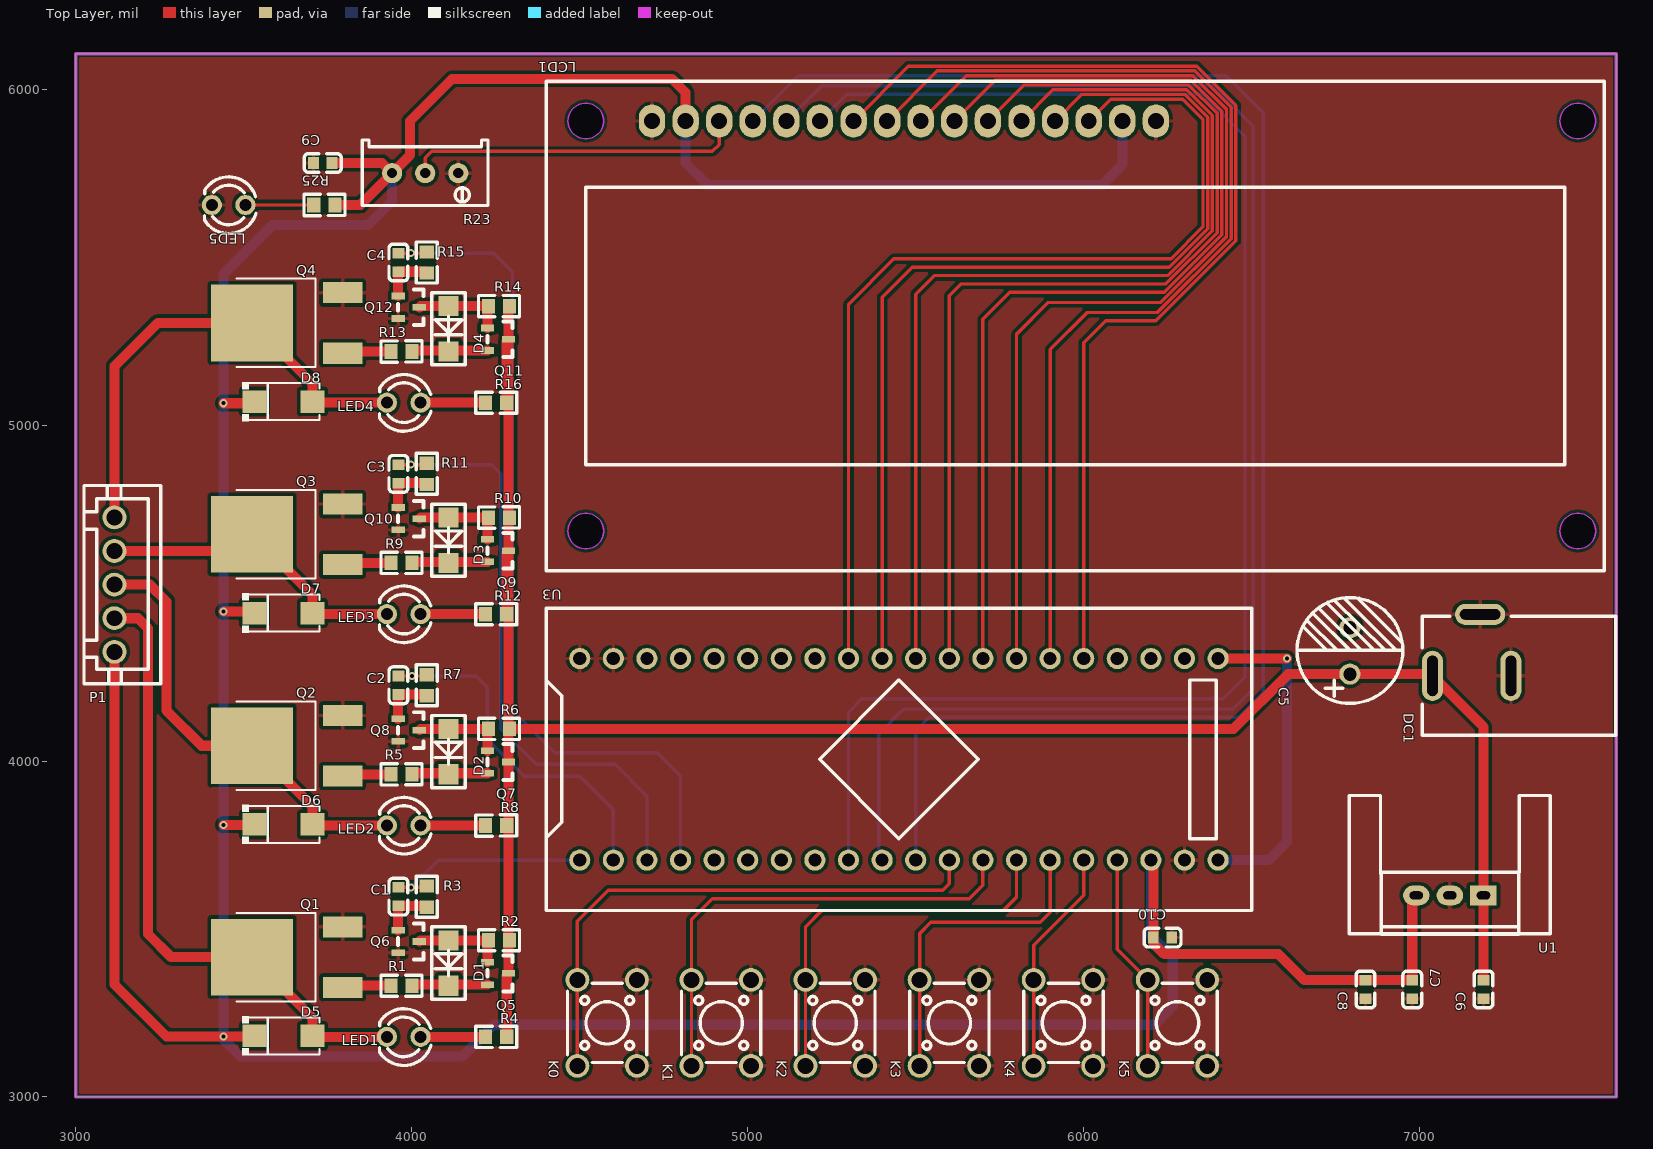
[diagram p0: Top Layer view]
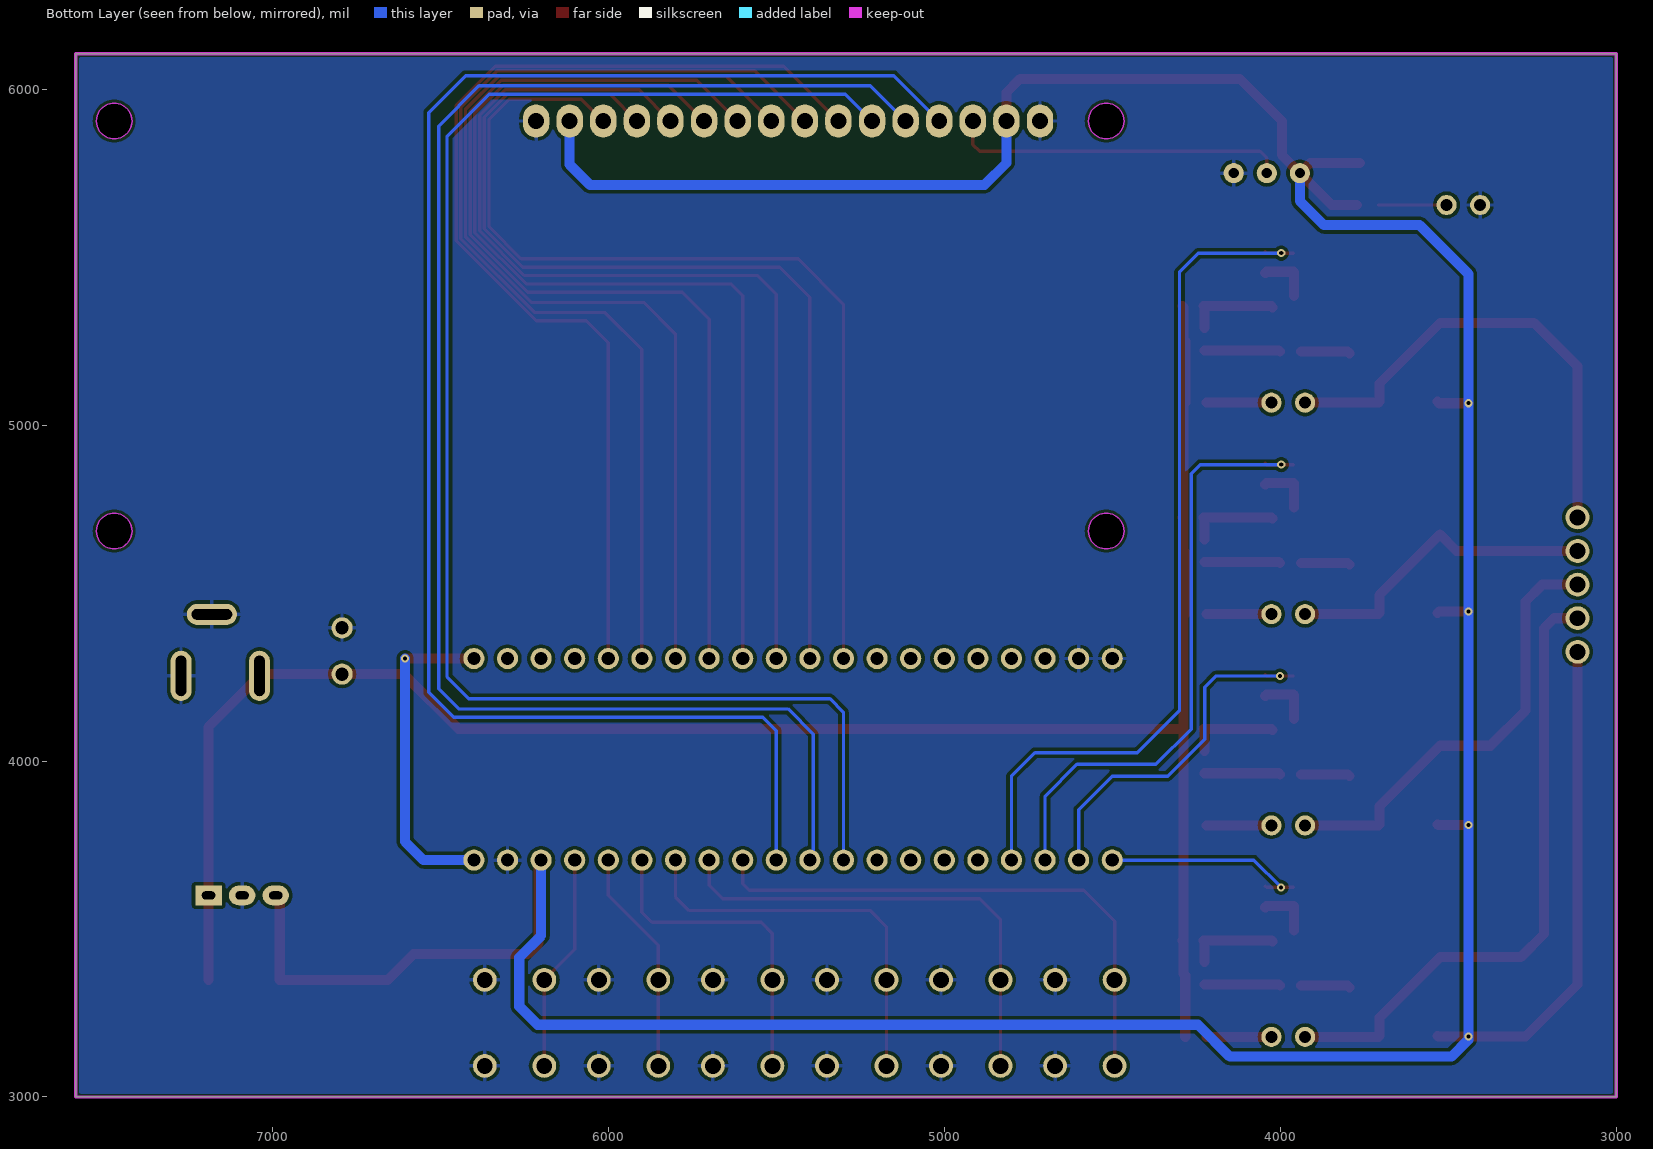
[diagram p1: Bottom Layer view, seen from below]
# Altium PCB MISC49935.pcbdoc
Units mil, origin at the board's own origin, x right, y up, seen from the top; angles counter-clockwise.
Board outline 4585 x 3105 mil, 2 copper layers (Top Layer, Bottom Layer), stack 62.206 mil thick; 64 components, 64 nets, 210 pads, 9 vias.

## Layer stack, top to bottom
Top Solder Mask Layer: solder mask 0.394, Dk 3.3
Top Layer: signal copper 1.379
Dielectric1: surface 59.449, FR4, Dk 4.5
Bottom Layer: signal copper 1.378
Bottom Solder Mask Layer: solder mask 0.394, Dk 3.3

## Board outline
3000,6105 3000,3000 7585,3000 7585,6105

## Design rules (kind name [scope] priority, off if disabled: settings)
BoardOutlineClearance copperThickness2oz_1 [All] p2 off: genericclearance=7.99 ignorepadtopadclearanceinfootprint=FALSE except(0: Arc-SplitContinuation Track-SplitContinuation SMDPad-SplitContinuation THPad-SplitContinuation Via-SplitContinuation Fill-SplitContinuation Region-SplitContinuation Poly-SplitContinuation Text-SplitContinuation Hole-SplitContinuation; 5.98: Arc-CutoutEdge SMDPad-CutoutEdge THPad-CutoutEdge Via-CutoutEdge Fill-CutoutEdge Region-CutoutEdge Text-CutoutEdge; 6.93: Hole-OutlineEdge Hole-CutoutEdge; 10: Poly-OutlineEdge Poly-CutoutEdge; 11.81: Arc-OutlineEdge Track-OutlineEdge SMDPad-OutlineEdge THPad-OutlineEdge Via-OutlineEdge Fill-OutlineEdge Region-OutlineEdge Text-OutlineEdge Track-CutoutEdge)
BoardOutlineClearance copperThickness1oz_1 [All] p4: genericclearance=4.02 ignorepadtopadclearanceinfootprint=FALSE except(0: Arc-SplitContinuation Track-SplitContinuation SMDPad-SplitContinuation THPad-SplitContinuation Via-SplitContinuation Fill-SplitContinuation Region-SplitContinuation Poly-SplitContinuation Text-SplitContinuation Hole-SplitContinuation; 6: SMDPad-CutoutEdge THPad-CutoutEdge Via-CutoutEdge Fill-CutoutEdge Region-CutoutEdge Text-CutoutEdge; 6.93: Hole-OutlineEdge Hole-CutoutEdge; 10: Poly-OutlineEdge Poly-CutoutEdge; 11.8: Arc-OutlineEdge Track-OutlineEdge SMDPad-OutlineEdge THPad-OutlineEdge Via-OutlineEdge Fill-OutlineEdge Region-OutlineEdge Text-OutlineEdge; 11.81: Arc-CutoutEdge Track-CutoutEdge)
Clearance copperThickness2oz [All] p1 off: gap=7.99 ignorepadtopadclearanceinfootprint=FALSE except(5.98: SMDPad-Track SMDPad-SMDPad THPad-Track SMDPad-THPad THPad-THPad Track-Via SMDPad-Via THPad-Via Via-Via Fill-Track Region-Track Fill-SMDPad Region-SMDPad Fill-THPad Region-THPad Fill-Via Region-Via Fill-Fill Fill-Region Region-Region Arc-Track Arc-SMDPad Arc-THPad Arc-Via Fill-Arc Region-Arc Arc-Arc Text-Track SMDPad-Text Text-THPad Text-Via Fill-Text Region-Text Arc-Text Text-Text; 6.93: Hole-Track Hole-SMDPad Hole-THPad Hole-Via Fill-Hole Region-Hole Hole-Arc Hole-Text; 10: Poly-Track Poly-SMDPad Poly-THPad Poly-Via Poly-Fill Poly-Region Poly-Poly Poly-Arc Poly-Text Poly-Hole)
Clearance copperThickness1oz [All] p3: gap=4.02 ignorepadtopadclearanceinfootprint=FALSE except(5.98: SMDPad-Track SMDPad-SMDPad THPad-Track SMDPad-THPad THPad-THPad Track-Via SMDPad-Via THPad-Via Via-Via Fill-Track Region-Track Fill-SMDPad Region-SMDPad Fill-THPad Region-THPad Fill-Via Region-Via Fill-Fill Fill-Region Region-Region; 6: Arc-Track Arc-SMDPad Arc-THPad Arc-Via Fill-Arc Region-Arc Arc-Arc Text-Track SMDPad-Text Text-THPad Text-Via Fill-Text Region-Text Arc-Text Text-Text; 6.93: Hole-Track Hole-SMDPad Hole-THPad Hole-Via Fill-Hole Region-Hole Hole-Arc Hole-Text; 10: Poly-Track Poly-SMDPad Poly-THPad Poly-Via Poly-Fill Poly-Region Poly-Poly Poly-Arc Poly-Text Poly-Hole)
Creepage creepage [All] p1: checkdistance=0 ignoreinternallayers=TRUE applytopolygonpour=TRUE
DiffPairsRouting differentialPair [All] p1: maxlimit=6 minlimit=6 mostfreqgap=6 toplayer_minwidth=5 toplayer_prefwidth=10 toplayer_maxwidth=100 toplayer_mingap=6 toplayer_prefgap=6 toplayer_maxgap=6 bottomlayer_minwidth=5 bottomlayer_prefwidth=10 bottomlayer_maxwidth=100 bottomlayer_mingap=6 bottomlayer_prefgap=6 bottomlayer_maxgap=6 maxuncoupledlength=10
HoleToHoleClearance otherClearance [All] p1: gap=11.81 allowstackedmicrovias=TRUE
Length netLength [All] p1: minlimit=0 maxlimit=0
MatchedLengths netLengthTolerance [All] p1: tolerance=1000
PasteMaskExpansion pasteMaskExpansion [All] p1: expansion=0
PlaneConnect innerPlane [All] p1: planeconnectstyle=Relief reliefexpansion=20 reliefentries=4 reliefconductorwidth=10 reliefairgap=10
PolygonConnect copperRegion [(InNet('GND'))] p1: connectstyle=Relief reliefconductorwidth=10 reliefentries=4 polygonreliefangle="90 Angle" airgapwidth=10 via.connectstyle=Relief via.reliefconductorwidth=10 via.reliefentries=4 via.polygonreliefangle="90 Angle" via.airgapwidth=10
RoutingVias viaSize [All] p1: holewidth=12.01 width=24.02 viastyle="Through Hole" minholewidth=11.81 minwidth=19.68 maxholewidth=248.03 maxwidth=393.7
SolderMaskExpansion solderMaskExpansion [IsVia] p1: expansion=-1000 istentingtop=TRUE
SolderMaskExpansion solderMaskExpansion [All] p2: expansion=2 istentingtop=FALSE
Width copperThickness2oz_2 [All] p1 off: maxlimit=100 minlimit=8 preferedwidth=10
Width copperThickness1oz_2 [All] p2: maxlimit=100 minlimit=5 preferedwidth=10

## Components (designator, comment, footprint, x,y, rotation, side; value= is the part's Value field where it differs from the comment)
C1 "1nF" C0603 3960.27,3596.17 r270 top
C2 "1nF" C0603 3960.27,4225.43 r270 top
C3 "1nF" C0603 3960.27,4854.68 r270 top
C4 "1nF" C0603 3960.27,5483.94 r270 top
C5 "470uF" 470uf 6795,4330 r90 top
C6 "100nF" C0603 7190,3320 r90 top
C7 "100uF" C0603 6978.03,3320 r270 top
C8 "100nF" C0603 6838.9,3320 r90 top
C9 "100nF" C0603 3735,5780 r0 top
C10 "100nF" C0603 6234.77,3474.49 r0 top
D1 "1N4148" 1N4148 4109.51,3401.21 r270 top
D2 "1N4148" 1N4148 4109.51,4030.47 r270 top
D3 "1N4148" 1N4148 4109.51,4659.72 r270 top
D4 "1N4148" 1N4148 4109.51,5288.98 r270 top
D5 "1N4007G" 1N4007G/M7 3616.09,3178.82 r0 top
D6 "1N4007G" 1N4007G/M7 3616.09,3808.08 r0 top
D7 "1N4007G" 1N4007G/M7 3616.09,4437.33 r0 top
D8 "1N4007G" 1N4007G/M7 3616.09,5066.59 r0 top
DC1 "EJ503A" DC-IN-TH_EJ503A 7155,4345 r90 top
K0 "Start/Stop" SW-TH_4P-L6.0-W6.0-P4.50-LS6.5 4581.56,3220.54 r90 top
K1 "Forward/Reverse" SW-TH_4P-L6.0-W6.0-P4.50-LS6.5 4921.09,3220.54 r90 top
K2 "Speed+10" SW-TH_4P-L6.0-W6.0-P4.50-LS6.5 5260.61,3220.54 r90 top
K3 "Speed+1" SW-TH_4P-L6.0-W6.0-P4.50-LS6.5 5600.14,3220.54 r90 top
K4 "Speed-10" SW-TH_4P-L6.0-W6.0-P4.50-LS6.5 5939.66,3220.54 r90 top
K5 "Speed-1" SW-TH_4P-L6.0-W6.0-P4.50-LS6.5 6279.19,3220.54 r90 top
LCD1 "LCM1602K-FSW-FBW-33V33" MODULE-TH_LCM1602K 5465,5905 r0 top
LED1 "3mmFIR" LED_TH-3mm 3976.09,3178.82 r180 top
LED2 "3mmFIR" LED_TH-3mm 3976.09,3808.08 r180 top
LED3 "3mmFIR" LED_TH-3mm 3976.09,4437.33 r180 top
LED4 "3mmFIR" LED_TH-3mm 3976.09,5066.59 r180 top
LED5 "3mmFIR" LED_TH-3mm 3455,5655 r180 top
P1 "Motor interface" CONN-TH_5P-P2.54_C9900008095 3115,4525 r90 top
Q1 "JSM80N03D" TO-252-2_L6.6-W6.1-P4.57-LS9.9-BR-CW 3659.51,3416.21 r0 top
Q2 "JSM80N03D" TO-252-2_L6.6-W6.1-P4.57-LS9.9-BR-CW 3659.51,4045.47 r0 top
Q3 "JSM80N03D" TO-252-2_L6.6-W6.1-P4.57-LS9.9-BR-CW 3659.51,4674.72 r0 top
Q4 "JSM80N03D" TO-252-2_L6.6-W6.1-P4.57-LS9.9-BR-CW 3659.51,5303.98 r0 top
Q5 "MMS9013-H-TP" MMS8050-H-TP 4225.27,3401.17 r270 top
Q6 "MMS9013-H-TP" MMS8050-H-TP 3959.51,3496.21 r270 top
Q7 "MMS9013-H-TP" MMS8050-H-TP 4225.27,4030.43 r270 top
Q8 "MMS9013-H-TP" MMS8050-H-TP 3959.51,4125.47 r270 top
Q9 "MMS9013-H-TP" MMS8050-H-TP 4225.27,4659.68 r270 top
Q10 "MMS9013-H-TP" MMS8050-H-TP 3959.51,4754.72 r270 top
Q11 "MMS9013-H-TP" MMS8050-H-TP 4225.27,5288.94 r270 top
Q12 "MMS9013-H-TP" MMS8050-H-TP 3959.51,5383.98 r270 top
R1 "5.1Ω" R0603 3969.51,3331.21 r180 top
R2 "10kΩ" R0603 4259.51,3466.21 r0 top
R3 "1kΩ" R0603 4044.51,3596.21 r270 top
R4 "10kΩ" R0603 4251.09,3178.82 r180 top
R5 "5.1Ω" R0603 3969.51,3960.47 r180 top
R6 "10kΩ" R0603 4259.51,4095.47 r0 top
R7 "1kΩ" R0603 4044.51,4225.47 r270 top
R8 "10kΩ" R0603 4251.09,3808.08 r180 top
R9 "5.1Ω" R0603 3969.51,4589.72 r180 top
R10 "10kΩ" R0603 4259.51,4724.72 r0 top
R11 "1kΩ" R0603 4044.51,4854.72 r270 top
R12 "10kΩ" R0603 4251.09,4437.33 r180 top
R13 "5.1Ω" R0603 3969.51,5218.98 r180 top
R14 "10kΩ" R0603 4259.51,5353.98 r0 top
R15 "1kΩ" R0603 4044.51,5483.98 r270 top
R16 "10kΩ" R0603 4251.09,5066.59 r180 top
R23 "10kΩ" R_3296 4040,5745 r180 top
R25 "3kΩ" R0603 3740,5655 r0 top
U1 "LM7805" LM7805 7090,3600 r180 top
U3 "LCKFB-DKX-STM32F103C8T6" CONN-TH_L53.3-W22.9_STM32F103C8T6-CARD 5450,4005 r0 top

## Footprints (in the part's own frame and the unit in brackets; to place one, negate y for a bottom-side part, rotate by r counter-clockwise, add the part's x,y. Pads: shape width x height; smd on the part's side, far side on the other; paste and mask are expansions set on the pad)
1N4007G/M7 [mm]
  rect 1.8x1.7 smd paste+0 mask+0.102: 1(-2.133,0.081) 2(2.252,0.081)
  silkscreen extent -3.05,-1.4 2.79,1.56
1N4148 [mil]
  rect 60x60 smd paste+0 mask+4: 1(70,0) 2(-65,0)
  silkscreen extent -105,-50 110,50
470uf [mm]
  round 1.6 hole 1 paste+0 mask+0.051: 1(-1.814,0.062) 2(1.686,0.062)
  silkscreen extent -4.03,-3.94 3.97,4.06
C0603 [mm]
  rect 0.8x0.9 smd: 1(-0.7,0) 2(0.7,0)
  silkscreen extent -1.39,-0.71 1.39,0.71
CONN-TH_5P-P2.54_C9900008095 [mm]
  round 1.8 hole 1.2 paste+0 mask+0.05: 1(-5.08,0) 2(-2.54,0) 3(0,0) 5(5.08,0)
  round 1.8 hole 1.2 copper offset 0,0 paste+0 mask+0.05: 4(2.54,0)
  silkscreen extent -7.5,-3.5 7.5,2.3
CONN-TH_L53.3-W22.9_STM32F103C8T6-CARD [mm]
  round 1.6 hole 1: 1(-24.13,-7.62) 2(-21.59,-7.62) 3(-19.05,-7.62) 4(-16.51,-7.62) 5(-13.97,-7.62) 6(-11.43,-7.62) 7(-8.89,-7.62) 8(-6.35,-7.62) 9(-3.81,-7.62) 10(-1.27,-7.62) 11(1.27,-7.62) 12(3.81,-7.62) 13(6.35,-7.62) 14(8.89,-7.62) 15(11.43,-7.62) 16(13.97,-7.62) 17(16.51,-7.62) 18(19.05,-7.62) 19(21.59,-7.62) 20(24.13,-7.62) 21(24.13,7.62) 22(21.59,7.62) 23(19.05,7.62) 24(16.51,7.62) 25(13.97,7.62) 26(11.43,7.62) 27(8.89,7.62) 28(6.35,7.62) 29(3.81,7.62) 30(1.27,7.62) 31(-1.27,7.62) 32(-3.81,7.62) 33(-6.35,7.62) 34(-8.89,7.62) 35(-11.43,7.62) 36(-13.97,7.62) 37(-16.51,7.62) 38(-19.05,7.62) 39(-21.59,7.62) 40(-24.13,7.62)
  silkscreen extent -26.67,-11.43 26.67,11.43
DC-IN-TH_EJ503A [mm]
  oval 3.8x1.6 hole 0.8 slot 3.05 at 0 deg paste+0 mask+0.05: 1(-2.325,2.965) 2(-2.325,-2.965)
  oval 1.6x3.8 hole 0.8 slot 3.05 at 90 deg copper offset 0,0 paste+0 mask+0.05: 3(2.325,-0.635)
  silkscreen extent -6.82,-10.89 2.18,3.73
LED_TH-3mm [mil]
  round 60 hole 36 paste+0 mask+2: 1(-50,0) 2(50,0)
  silkscreen extent -81,-84 72,85
LM7805 [mm]
  rect 2x1.5 hole 0.6 slot 1 at 0 deg: 1(-2.54,0)
  oval 2x1.5 hole 0.6 slot 1 at 0 deg: 2(0,0) 3(2.54,0)
  silkscreen extent -7.6,-7.55 7.6,2.95
MMS8050-H-TP [mm]
  rect 0.5x1 smd paste+0 mask+0.102: 1(0,0) 2(1.7,0) 3(0.85,1.6)
  silkscreen extent -0.5,0 2.2,1.9
MODULE-TH_LCM1602K [mm]
  oval 2x2.5 hole 1.2: 1(-19.05,0) 2(-16.51,0) 3(-13.97,0) 4(-11.43,0) 5(-8.89,0) 6(-6.35,0) 7(-3.81,0) 8(-1.27,0) 9(1.27,0) 10(3.81,0) 11(6.35,0) 12(8.89,0) 13(11.43,0) 14(13.97,0) 15(16.51,0) 16(19.05,0)
  Board Outline Layer circle w0.003: c-24.051,0 r1.35
  Board Outline Layer circle w0.003: c50.95,0 r1.35
  Board Outline Layer circle w0.003: c50.95,-31.001 r1.35
  Board Outline Layer circle w0.003: c-24.051,-31.001 r1.35
  Board Outline Layer region: -22.701,0 -22.835,-0.586 -23.21,-1.055 -23.751,-1.316 -24.352,-1.316 -24.893,-1.055 -25.268,-0.586 -25.401,0 -25.401,0 -25.268,0.586 -24.893,1.055 -24.352,1.316 -23.751,1.316 -23.21,1.055 -22.835,0.586 -22.701,0
  Board Outline Layer region: -22.701,0 -22.711,-0.163 -22.74,-0.323 -22.789,-0.479 -22.856,-0.627 -22.94,-0.767 -23.041,-0.895 -23.156,-1.01 -23.284,-1.111 -23.424,-1.195 -23.573,-1.262 -23.728,-1.311 -23.889,-1.34 -24.051,-1.35 -24.214,-1.34 -24.374,-1.311 -24.53,-1.262 -24.679,-1.195 -24.818,-1.111 -24.946,-1.01 -25.062,-0.895 -25.162,-0.767 -25.247,-0.627 -25.314,-0.479 -25.362,-0.323 -25.391,-0.163 -25.401,0 -25.391,0.163 -25.362,0.323 -25.314,0.479 -25.247,0.627 -25.162,0.767 -25.062,0.895 -24.946,1.01 -24.818,1.111 -24.679,1.195 -24.53,1.262 -24.374,1.311 -24.214,1.34 -24.051,1.35 -23.889,1.34 -23.728,1.311 -23.573,1.262 -23.424,1.195 -23.284,1.111 -23.156,1.01 -23.041,0.895 -22.94,0.767 -22.856,0.627 -22.789,0.479 -22.74,0.323 -22.711,0.163
  Board Outline Layer region: 52.3,0 52.166,-0.586 51.792,-1.055 51.25,-1.316 50.649,-1.316 50.108,-1.055 49.734,-0.586 49.6,0 49.6,0 49.734,0.586 50.108,1.055 50.649,1.316 51.25,1.316 51.792,1.055 52.166,0.586 52.3,0
  Board Outline Layer region: 52.3,0 52.29,-0.163 52.261,-0.323 52.212,-0.479 52.145,-0.627 52.061,-0.767 51.96,-0.895 51.845,-1.01 51.717,-1.111 51.577,-1.195 51.429,-1.262 51.273,-1.311 51.113,-1.34 50.95,-1.35 50.787,-1.34 50.627,-1.311 50.471,-1.262 50.322,-1.195 50.183,-1.111 50.055,-1.01 49.939,-0.895 49.839,-0.767 49.754,-0.627 49.688,-0.479 49.639,-0.323 49.61,-0.163 49.6,0 49.61,0.163 49.639,0.323 49.688,0.479 49.754,0.627 49.839,0.767 49.939,0.895 50.055,1.01 50.183,1.111 50.322,1.195 50.471,1.262 50.627,1.311 50.787,1.34 50.95,1.35 51.113,1.34 51.273,1.311 51.429,1.262 51.577,1.195 51.717,1.111 51.845,1.01 51.96,0.895 52.061,0.767 52.145,0.627 52.212,0.479 52.261,0.323 52.29,0.163
  Board Outline Layer region: 52.3,-31.001 52.166,-31.586 51.792,-32.056 51.25,-32.317 50.649,-32.317 50.108,-32.056 49.734,-31.586 49.6,-31.001 49.6,-31.001 49.734,-30.415 50.108,-29.945 50.649,-29.685 51.25,-29.685 51.792,-29.945 52.166,-30.415 52.3,-31.001
  Board Outline Layer region: 52.3,-31.001 52.29,-31.163 52.261,-31.324 52.212,-31.479 52.145,-31.628 52.061,-31.768 51.96,-31.896 51.845,-32.011 51.717,-32.112 51.577,-32.196 51.429,-32.263 51.273,-32.311 51.113,-32.341 50.95,-32.351 50.787,-32.341 50.627,-32.311 50.471,-32.263 50.322,-32.196 50.183,-32.112 50.055,-32.011 49.939,-31.896 49.839,-31.768 49.754,-31.628 49.688,-31.479 49.639,-31.324 49.61,-31.163 49.6,-31.001 49.61,-30.838 49.639,-30.678 49.688,-30.522 49.754,-30.373 49.839,-30.234 49.939,-30.105 50.055,-29.99 50.183,-29.89 50.322,-29.805 50.471,-29.738 50.627,-29.69 50.787,-29.661 50.95,-29.651 51.113,-29.661 51.273,-29.69 51.429,-29.738 51.577,-29.805 51.717,-29.89 51.845,-29.99 51.96,-30.105 52.061,-30.234 52.145,-30.373 52.212,-30.522 52.261,-30.678 52.29,-30.838
  Board Outline Layer region: -22.701,-31.001 -22.835,-31.586 -23.21,-32.056 -23.751,-32.317 -24.352,-32.317 -24.893,-32.056 -25.268,-31.586 -25.401,-31.001 -25.401,-31.001 -25.268,-30.415 -24.893,-29.945 -24.352,-29.685 -23.751,-29.685 -23.21,-29.945 -22.835,-30.415 -22.701,-31.001
  Board Outline Layer region: -22.701,-31.001 -22.711,-31.163 -22.74,-31.324 -22.789,-31.479 -22.856,-31.628 -22.94,-31.768 -23.041,-31.896 -23.156,-32.011 -23.284,-32.112 -23.424,-32.196 -23.573,-32.263 -23.728,-32.311 -23.889,-32.341 -24.051,-32.351 -24.214,-32.341 -24.374,-32.311 -24.53,-32.263 -24.679,-32.196 -24.818,-32.112 -24.946,-32.011 -25.062,-31.896 -25.162,-31.768 -25.247,-31.628 -25.314,-31.479 -25.362,-31.324 -25.391,-31.163 -25.401,-31.001 -25.391,-30.838 -25.362,-30.678 -25.314,-30.522 -25.247,-30.373 -25.162,-30.234 -25.062,-30.105 -24.946,-29.99 -24.818,-29.89 -24.679,-29.805 -24.53,-29.738 -24.374,-29.69 -24.214,-29.661 -24.051,-29.651 -23.889,-29.661 -23.728,-29.69 -23.573,-29.738 -23.424,-29.805 -23.284,-29.89 -23.156,-29.99 -23.041,-30.105 -22.94,-30.234 -22.856,-30.373 -22.789,-30.522 -22.74,-30.678 -22.711,-30.838
  Multi-Layer board cut-out: -22.701,0 -22.835,-0.586 -23.21,-1.055 -23.751,-1.316 -24.352,-1.316 -24.893,-1.055 -25.268,-0.586 -25.401,0 -25.401,0 -25.268,0.586 -24.893,1.055 -24.352,1.316 -23.751,1.316 -23.21,1.055 -22.835,0.586 -22.701,0
  Multi-Layer board cut-out: 52.3,0 52.166,-0.586 51.792,-1.055 51.25,-1.316 50.649,-1.316 50.108,-1.055 49.734,-0.586 49.6,0 49.6,0 49.734,0.586 50.108,1.055 50.649,1.316 51.25,1.316 51.792,1.055 52.166,0.586 52.3,0
  Multi-Layer board cut-out: 52.3,-31.001 52.166,-31.586 51.792,-32.056 51.25,-32.317 50.649,-32.317 50.108,-32.056 49.734,-31.586 49.6,-31.001 49.6,-31.001 49.734,-30.415 50.108,-29.945 50.649,-29.685 51.25,-29.685 51.792,-29.945 52.166,-30.415 52.3,-31.001
  Multi-Layer board cut-out: -22.701,-31.001 -22.835,-31.586 -23.21,-32.056 -23.751,-32.317 -24.352,-32.317 -24.893,-32.056 -25.268,-31.586 -25.401,-31.001 -25.401,-31.001 -25.268,-30.415 -24.893,-29.945 -24.352,-29.685 -23.751,-29.685 -23.21,-29.945 -22.835,-30.415 -22.701,-31.001
  silkscreen extent -27.05,-34 52.95,3
R0603 [mm]
  rect 1x1.1 smd paste+0 mask+0.102: 1(-0.8,0) 2(0.8,0)
  silkscreen extent -1.55,-0.8 1.55,0.81
R_3296 [mil]
  round 60 hole 30 paste+0 mask+2: 1(-98.4,-5) 2(0,-5) 3(98.4,-5)
  silkscreen extent -187,-103 187,92
SW-TH_4P-L6.0-W6.0-P4.50-LS6.5 [mm]
  round 1.8 hole 1.2: 1(-3.25,2.25) 2(3.25,2.25) 3(-3.25,-2.25) 4(3.25,-2.25)
  silkscreen extent -3,-3 3,3
TO-252-2_L6.6-W6.1-P4.57-LS9.9-BR-CW [mm]
  rect 3x1.6 smd: 1(3.424,-2.29) 3(3.424,2.29)
  rect 6.2x5.8 smd: 2(-3.424,0)
  silkscreen extent -4.58,-3.35 1.38,3.35

## Via types
v1: diameter 24.02, hole 12, Top Layer to Bottom Layer, 9 vias

## Nets (pads, with @x,y where several pads share a name; then routed paths per layer and width w, separated by ;. In a path a pad name is that pad's centre, name@x,y a point inside that pad or via, vN(x,y) a via of type N, cw(c..) or ccw(c..) an arc to the next point about the centre after c; other vN are vias at no path point)
$1N1: D6.2 LED2.2 P1.3 Q2.2 | length 1330.2
  Top Layer w30: P1.3 3220,4525 3270,4475 3270,4150 3374.53,4045.47 Q2.2 3704.74,3865.43 D6.2 3707.91,3808.08 LED2.2
$1N3: D5.2 LED1.2 P1.2 Q1.2 | length 1892.1
  Top Layer w30: P1.2 3185,4425 3215,4395 3215,3485 3283.79,3416.21 Q1.2 3704.74,3236.17 D5.2 3707.91,3178.82 LED1.2
$1N6: D7.2 LED3.2 P1.4 Q3.2 | length 961.8
  Top Layer w30: P1.4 3474.99,4625.01 Q3.2 3704.74,4494.68 D7.2 3707.91,4437.33 LED3.2
$1N8: D8.2 LED4.2 P1.5 Q4.2 | length 1444.6
  Top Layer w30: P1.5 3115,5175 3243.98,5303.98 Q4.2 3704.74,5123.94 D8.2 3707.91,5066.59 LED4.2
$1N9: Q1.1 R1.2 | length 145.8
  Top Layer w30: Q1.1 3799.47,3331.21 R1.2
$1N10: LED1.1 R4.2 | length 193.5
  Top Layer w30: LED1.1 R4.2
$1N12: D1.1 Q5.2 R1.1 | length 225.5
  Top Layer w30: R1.1 4004.03,3334.24 Q5.2
$1N13: D1.2 Q5.1 Q6.3 R2.1 | length 273.1
  Top Layer w30: Q6.3 4025.96,3466.21 D1.2 R2.1 4225.27,3463.46 Q5.1
$1N15: C1.2 Q6.1 R3.2 | length 158.6
  Top Layer w30: Q6.1 3959.51,3567.85 C1.2 4040.6,3568.61 R3.2
$1N18: C2.2 Q8.1 R7.2 | length 158.6
  Top Layer w30: Q8.1 3959.51,4197.11 C2.2 4040.6,4197.87 R7.2
$1N20: D2.2 Q7.1 Q8.3 R6.1 | length 273.1
  Top Layer w30: Q8.3 4025.96,4095.47 D2.2 R6.1 4225.27,4092.72 Q7.1
$1N21: D2.1 Q7.2 R5.1 | length 225.5
  Top Layer w30: R5.1 4004.03,3963.5 Q7.2
$1N23: LED2.1 R8.2 | length 193.5
  Top Layer w30: LED2.1 R8.2
$1N24: Q2.1 R5.2 | length 145.8
  Top Layer w30: Q2.1 3799.47,3960.47 R5.2
$1N26: C3.2 Q10.1 R11.2 | length 158.6
  Top Layer w30: Q10.1 3959.51,4826.36 C3.2 4040.6,4827.12 R11.2
$1N28: D3.2 Q9.1 Q10.3 R10.1 | length 273.1
  Top Layer w30: Q10.3 4025.96,4724.72 D3.2 R10.1 4225.27,4721.97 Q9.1
$1N29: D3.1 Q9.2 R9.1 | length 225.5
  Top Layer w30: R9.1 4004.03,4592.75 Q9.2
$1N31: LED3.1 R12.2 | length 193.5
  Top Layer w30: LED3.1 R12.2
$1N32: Q3.1 R9.2 | length 145.8
  Top Layer w30: Q3.1 3799.47,4589.72 R9.2
$1N34: C4.2 Q12.1 R15.2 | length 158.6
  Top Layer w30: Q12.1 3959.51,5455.62 C4.2 4040.6,5456.38 R15.2
$1N36: D4.2 Q11.1 Q12.3 R14.1 | length 273.1
  Top Layer w30: Q12.3 4025.96,5353.98 D4.2 R14.1 4225.27,5351.23 Q11.1
$1N37: D4.1 Q11.2 R13.1 | length 225.5
  Top Layer w30: R13.1 4004.03,5222.01 Q11.2
$1N39: LED4.1 R16.2 | length 193.5
  Top Layer w30: LED4.1 R16.2
$1N40: Q4.1 R13.2 | length 145.8
  Top Layer w30: Q4.1 3799.47,5218.98 R13.2
$1N44: LCD1.3 R23.2 | length 1006.6
  Top Layer w10: R23.2 4040,5795 4060,5815 4895,5815 4915,5835 LCD1.3
$1N59: LED5.1 R25.1 | length 203.5
  Top Layer w10: LED5.1 R25.1
$1N63: U3.22
$1N65: U3.23
$1N66: U3.24
$1N84: U3.33
$1N85: U3.8
$1N86: U3.34
$1N87: U3.7
$1N88: U3.35
$1N89: U3.6
$1N90: U3.36
$1N91: U3.5
$1N92: U3.37
$1N94: U3.38
+3.3V: U3.20 U3.21 | length 977.8
  Top Layer w30: U3.21 v1(6605,4305)
  Bottom Layer w30: U3.20 6550,3705 6605,3760 v1(6605,4305)
+5V: C7.1 C8.2 C9.2 C10.1 D5.1 D6.1 D7.1 D8.1 LCD1.2 LCD1.15 P1.1 R23.3 R25.2 U1.3 U3.18 | length 12559.5
  Top Layer w30: P1.1 3115,3335 3270,3180 v1(3440,3180) 3530.12,3180 D5.1 ; v1(3440,3810) 3530.86,3810 D6.1 ; v1(3440,4445) 3527.61,4445 D7.1 ; v1(3440,5065) 3527.35,5065 D8.1 ; C9.2 3911.6,5780 R23.3 ; R25.2 3846.6,5655 R23.3 ; LCD1.2 4815,5990 4775,6030 4120,6030 3995,5905 3995,5803.4 R23.3 ; U3.18 6207.2,3697.8 C10.1 6207.2,3457.8 6240,3425 6580,3425 6657.44,3347.56 C8.2 C7.1 6978.03,3588.03 U1.3
  Bottom Layer w30: R23.3 3941.6,5666.6 3870,5595 3585,5595 3440,5450 v1(3440,5065) v1(3440,4445) v1(3440,3810) 3440,3170 3490,3120 4150,3120 4245,3215 6210,3215 6265,3270 6265,3415 6200,3480 U3.18 ; LCD1.2 4815,5780 4880,5715 6055,5715 6115,5775 LCD1.15
+12V: C5.1 C6.2 DC1.1 Q5.3 Q7.3 Q9.3 Q11.3 R2.2 R4.1 R6.2 R8.1 R10.2 R12.1 R14.2 R16.1 U1.1 | length 6354.6
  Top Layer w30: R4.1 4282.58,3362.03 Q5.3 R2.2@4288.26,3463.46 ; R12.1 4282.58,4620.54 Q9.3 ; R16.1 4282.58,5249.8 Q11.3 ; R2.2 R2.2@4288.26,3463.46 ; R6.2 6445.47,4095.47 6608.58,4258.58 C5.1 7033.15,4258.58 DC1.1 7190,4101.73 U1.1 C6.2 ; R10.2 R10.2@4288.26,4721.98 ; R14.2 4288.26,5351.23 Q11.3 ; R2.2@4288.26,3463.46 Q7.3 Q9.3 ; Q9.3 R10.2@4288.26,4721.98 ; R10.2@4288.26,4721.98 Q11.3
GND: C5.2 C6.1 C7.2 C8.1 C9.1 C10.2 DC1.2 DC1.3 K0.3 K0.4 K1.3 K1.4 K2.3 K2.4 K3.3 K3.4 K4.3 K4.4 K5.3 K5.4 LCD1.1 LCD1.16 LED5.2 Q1.3 Q2.3 Q3.3 Q4.3 Q6.2 Q8.2 Q10.2 Q12.2 R23.1 U1.2 U3.19 U3.39 U3.40
K0: K0.1 K0.2 U3.12 | length 1653.8
  Top Layer w10: K0.1 K0.2 4492.98,3522.98 4585,3615 5580,3615 5600,3635 U3.12
K1: K1.1 K1.2 U3.13 | length 1419.9
  Top Layer w10: K1.1 K1.2 4832.51,3527.51 4895,3590 5660,3590 5700,3630 U3.13
K2: K2.1 K2.2 U3.14 | length 1188.8
  Top Layer w10: K2.1 K2.2 5172.03,3507.03 5220,3555 5760,3555 5800,3595 U3.14
K3: K3.1 K3.2 U3.15 | length 963.7
  Top Layer w10: K3.1 K3.2 5511.56,3486.56 5545,3520 5870,3520 5900,3550 U3.15
K4: K4.1 K4.2 U3.16 | length 674.1
  Top Layer w10: K4.1 K4.2 5851.09,3451.09 6000,3600 U3.16
K5: K5.1 K5.2 U3.17 | length 649.9
  Top Layer w10: U3.17 6100,3439.1 K5.2 K5.1
"LCD DB0": LCD1.7 U3.25 | length 3175.6
  Top Layer w10: LCD1.7 5478.11,6068.11 6336.35,6068.11 6453.11,5951.35 6453.11,5548.65 6214.46,5310 6065,5310 6000,5245 U3.25
"LCD DB1": LCD1.8 U3.26 | length 3117.5
  Top Layer w10: LCD1.8 5564.09,6054.09 6330.55,6054.09 6439.09,5945.55 6439.09,5554.45 6219.64,5335 6010,5335 5900,5225 U3.26
"LCD DB2": LCD1.9 U3.27 | length 3097.4
  Top Layer w10: LCD1.9 5650.08,6040.08 6324.74,6040.08 6425.08,5939.74 6425.08,5560.26 6229.82,5365 5895,5365 5800,5270 U3.27
"LCD DB3": LCD1.10 U3.28 | length 3077.3
  Top Layer w10: LCD1.10 5736.06,6026.06 6318.94,6026.06 6411.06,5933.94 6411.06,5566.06 6240,5395 5780,5395 5700,5315 U3.28
"LCD DB4": LCD1.11 U3.29 | length 3071
  Top Layer w10: U3.29 5600,5385 5635,5420 6244.46,5420 6397.05,5572.58 6397.05,5927.42 6312.42,6012.05 5822.05,6012.05 LCD1.11
"LCD DB5": LCD1.12 U3.30 | length 3027.5
  Top Layer w10: U3.30 5500,5390 5555,5445 6249.64,5445 6383.03,5578.39 6383.03,5921.61 6306.61,5998.03 5908.03,5998.03 LCD1.12
"LCD DB6": LCD1.13 U3.31 | length 2975.2
  Top Layer w10: U3.31 5400,5380 5490,5470 6254.82,5470 6369.02,5584.19 6369.02,5915.81 6300.81,5984.02 5994.02,5984.02 LCD1.13
"LCD DB7": LCD1.14 U3.32 | length 2917
  Top Layer w10: U3.32 5300,5360 5435,5495 6260,5495 6355,5590 6355,5910 6295,5970 6080,5970 LCD1.14
"LCD E": LCD1.6 U3.9 | length 4623.4
  Bottom Layer w10: LCD1.6 5295,5985 6355,5985 6480,5860 6480,4250 6415,4185 5340,4185 5300,4145 U3.9
"LCD RS": LCD1.4 U3.11 | length 4814.1
  Bottom Layer w10: LCD1.4 5150,6040 6425,6040 6535,5930 6535,4205 6460,4130 5540,4130 5500,4090 U3.11
"LCD RW": LCD1.5 U3.10 | length 4708.3
  Bottom Layer w10: LCD1.5 5220,6010 6385,6010 6505,5890 6505,4215 6445,4155 5465,4155 5390,4080 5390,3715 U3.10
"MT A": C1.1 R3.1 U3.1 | length 622.1
  Top Layer w10: C1.1 v1(3997.41,3623.73) 4040.54,3623.73 R3.1
  Bottom Layer w10: v1(3997.41,3623.73) 4078.68,3705 U3.1
"MT B": C2.1 R7.1 U3.2 | length 1091.2
  Top Layer w10: C2.1 v1(4000.35,4252.99) 4040.54,4252.99 R7.1
  Bottom Layer w10: v1(4000.35,4252.99) 4192.01,4252.99 4225,4220 4225,4065 4335,3955 4500,3955 4600,3855 U3.2
"MT C": C3.1 R11.1 U3.3 | length 1833
  Top Layer w10: C3.1 v1(3996.98,4882.24) 4040.54,4882.24 R11.1
  Bottom Layer w10: v1(3996.98,4882.24) 4237.76,4882.24 4265,4855 4265,4095 4370,3990 4605,3990 4700,3895 U3.3
"MT D": C4.1 R15.1 U3.4 | length 2548.1
  Top Layer w10: C4.1 v1(3996.94,5511.5) 4040.54,5511.5 R15.1
  Bottom Layer w10: v1(3996.94,5511.5) 4243.5,5511.5 4300,5455 4300,4150 4425,4025 4730,4025 4800,3955 U3.4

## Polygon pours and split planes (outlines as drawn)
GND on Top Layer (solid, remove dead copper, pour order 0): 3000,6105 3000,3000 7585,3000 7585,6105
GND on Bottom Layer (solid, remove dead copper, pour order 2): 3000,6105 3000,3000 7585,3000 7585,6105

## Keep-outs
Board Outline Layer:
  the board outline again, w10